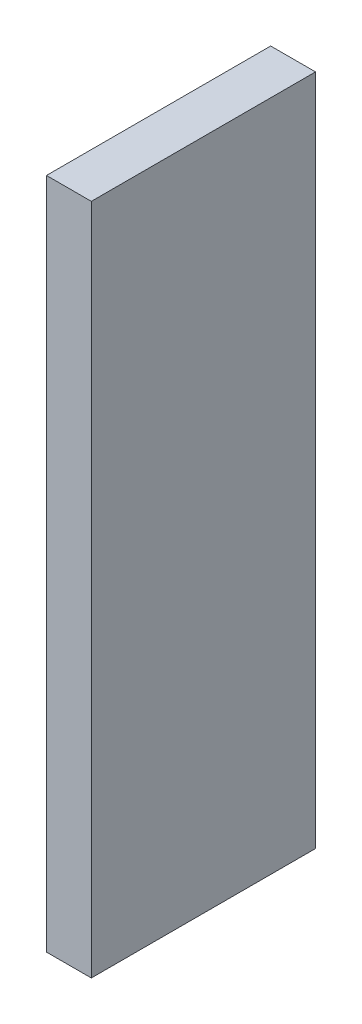
SolidWorks part; units mm, degrees
material "Q235"
ref_plane "前视基准面" through (0, 0, 0) normal (0, 0, 1) x (1, 0, 0)
ref_plane "上视基准面" through (0, 0, 0) normal (0, 1, 0) x (1, 0, 0)
ref_plane "右视基准面" through (0, 0, 0) normal (1, 0, 0) x (0, 0, -1)
sketch "草图1" plane through (0, 0, 0) normal (1, 0, 0) x (0, 0, -1)
  line L1 (0, 0) -> (20, 0)
  line L2 (0, 0) -> (0, 60)
  line L3 (0, 60) -> (20, 60)
  line L4 (20, 0) -> (20, 60)
  dimension "D1" = 20
  dimension "D2" = 60
extrude "凸台-拉伸1" add sketch "草图1" along normal blind 4
